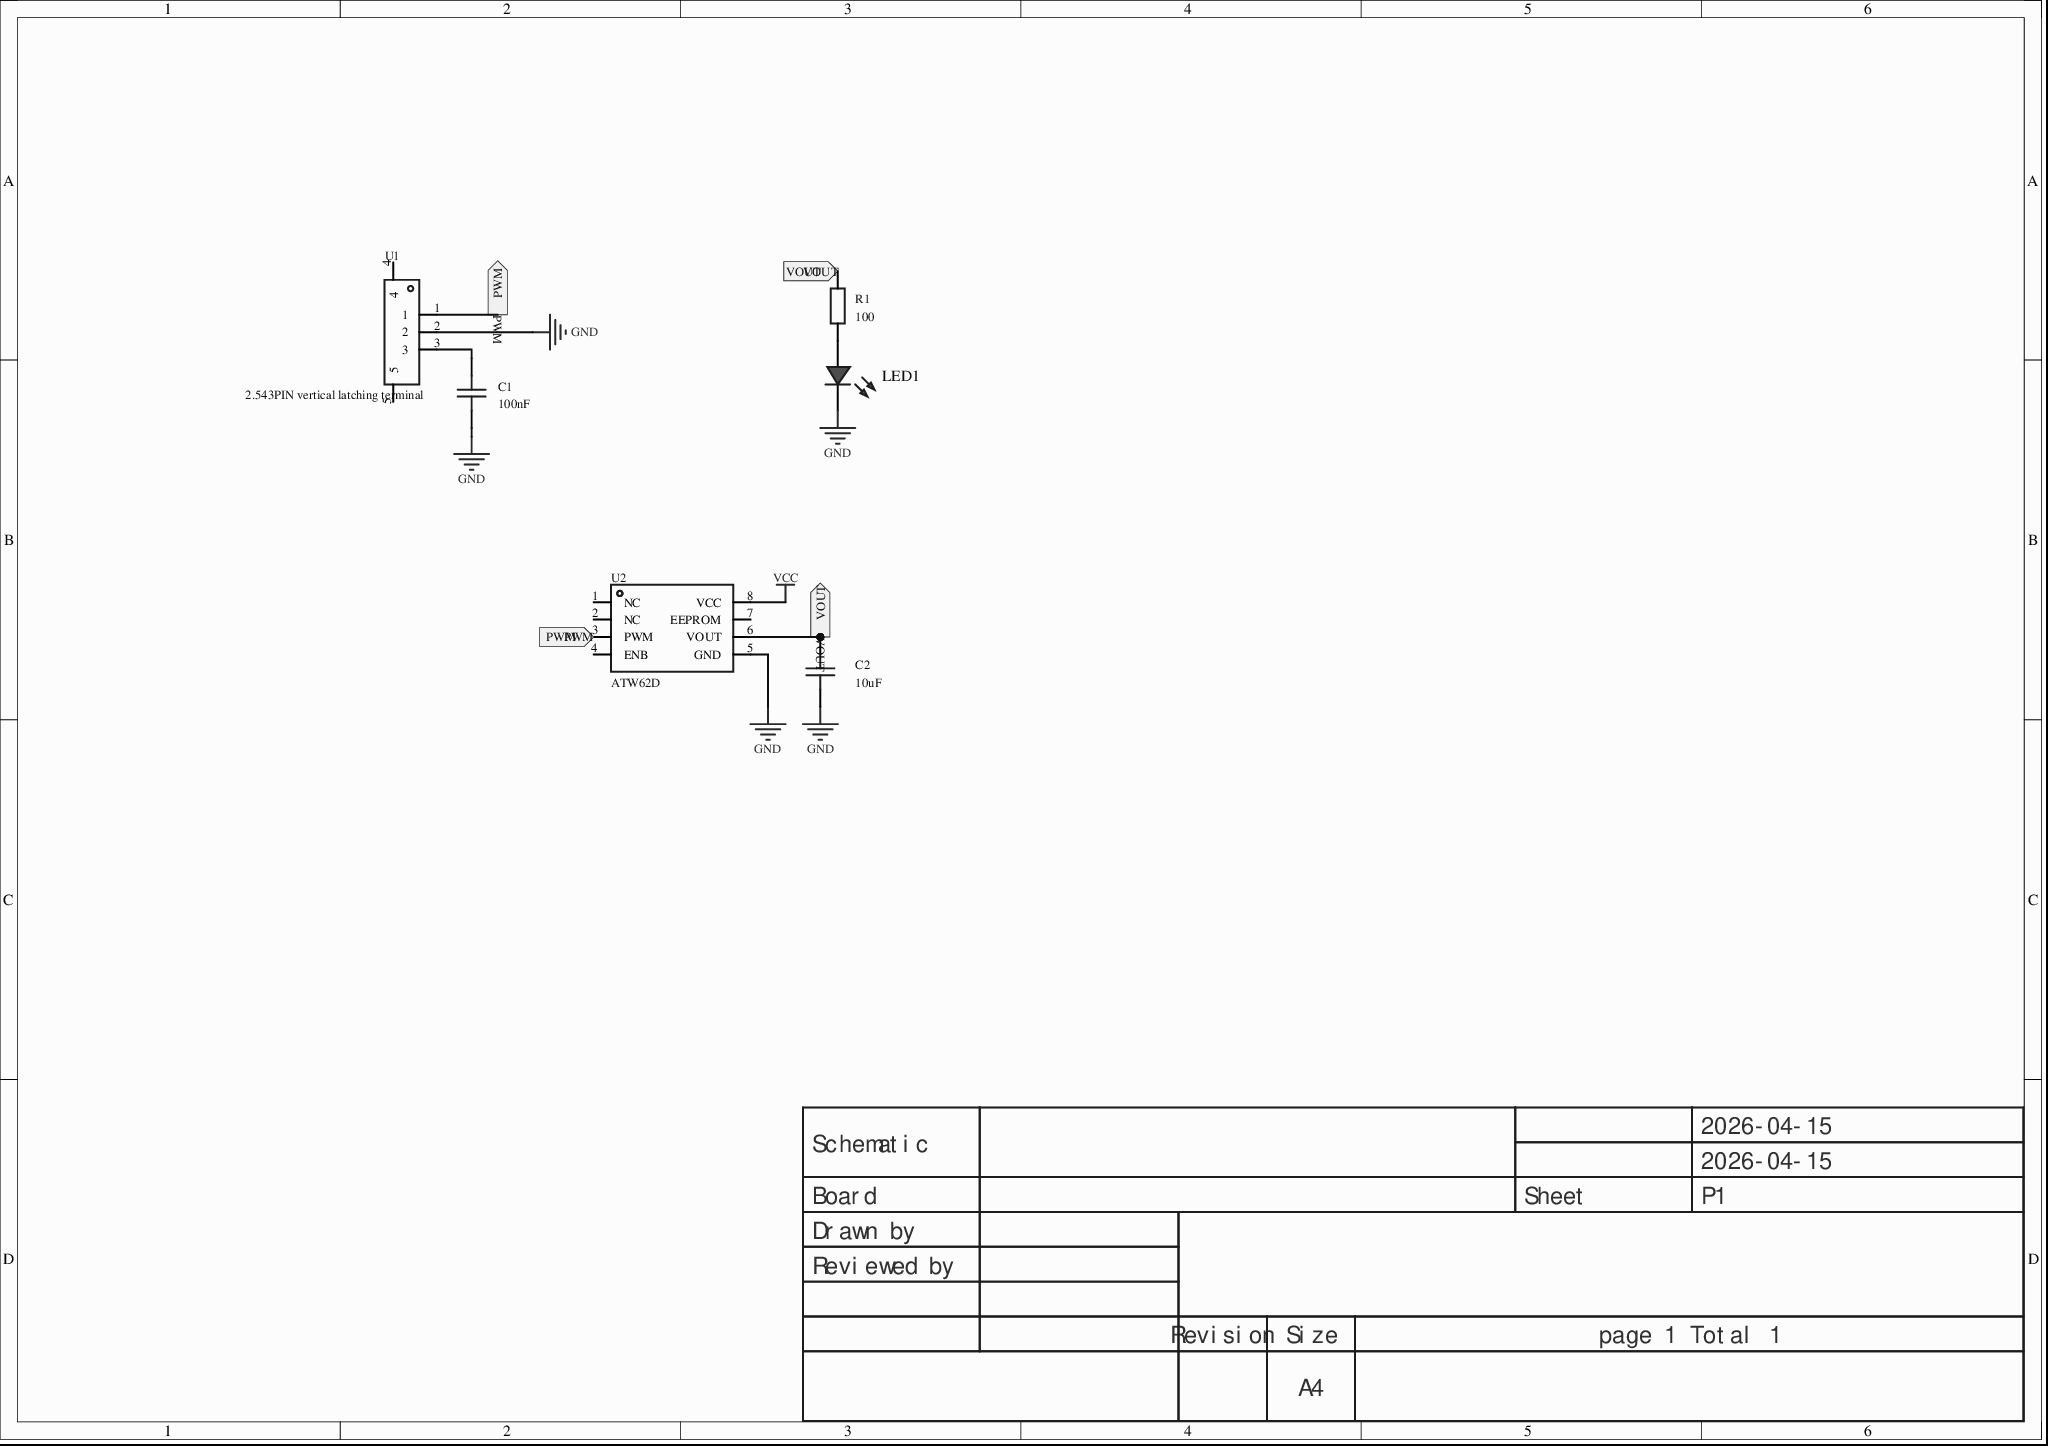
[diagram p0: MISC51135-3.schdoc]
# Altium project MISC51135-2.PrjPcb
1 sheet, 6 parts. Net scope: flat (ports and power ports of the same name join across sheets).
Board file: MISC51135.pcbdoc

## Sheet MISC51135-3.schdoc
size 297 x 209 mm; Version: V1.0; @Project Name: MISC51135; @Update Date: 2026-04-15; @Create Date: 2026-04-15; @Board Name: MISC51135; @Create Time: 19:41:14; @Page Count: 1; @Page No: 1; @Schematic Name: MISC51135; @Update Time: 19:41:14; Size: A4

### Parts
C1  100nF  [C0603]
C2  10uF  [C0603]
LED1  (no value)  [LED_0603]
R1  100  [R0603]
U1  2.543PIN vertical latching terminal  [CONN-SMD_3P-P2.54_C9900012759]
U2  ATW62D  [SOP-8_L4.9-W3.9-P1.27-LS6.0-TL]

### Ports
PWM (in), PWM (out), VOUT (in), VOUT (out)

### Nets
GND: C1.1 C2.1 LED1.1(C) U1.2 U2.5(GND)
VCC: U2.8(VCC)
PWM: U1.1 U2.3(PWM) ; port PWM
VOUT: C2.2 R1.2 U2.6(VOUT) ; port VOUT
NetC1_2: C1.2 U1.3
NetLED1_2: LED1.2(A) R1.1

Not connected (* = marked no-connect by the designer): U1 4 5; U2 1(NC)* 2(NC)* 4(ENB)* 7(EEPROM)*

### Notes on the sheet
- 2026-04-15
- Schematic
- Board
- Sheet
- P1
- Drawn by
- Reviewed by
- Revision
- Size
- A4
- page 1 Total 1

### Library data of the parts
C1 C2 = CAP_0603: Symbol: Capacitance; ConvertToPcb: yes; ModelId: ac125912035d415993ca9572d50418b10819f05c4eef4c71ace90d822a990e87; ModelName: C0603_L1.6-W0.8-H0.8; ModelTransform: 62.992,31.496,0,0,0,0,0,0,0; Device: CAP_0603; AddInBom: yes; Supplier Footprint: 0603; FootprintName: C0603
  C1: Value: 100nF
  C2: Value: 10uF
LED1 = LED_0603-R: Symbol: LED_R; Convert to PCB: yes; 3D Model: dd8257b0d61a4cd7b68939a056e080950819f05c4eef4c71ace90d822a990e87; 3D Model Transform: 58.72,29.4,22.03,0,0,0,0,0,0; ModelName: LED-0603_R; Device: LED_0603-R; Add into BOM: yes; Supplier Footprint: 0603; FootprintName: LED_0603
R1 = Res_0603: Symbol: Resistor; ConvertToPcb: yes; ModelId: fc143cca1e79419f9cd78b61e9279f080819f05c4eef4c71ace90d822a990e87; ModelTransform: 31.8897,63.7794,0,90,0,0,0,0,0; Device: Res_0603; Value: 100; AddInBom: yes; Supplier Footprint: 0603; FootprintName: R0603; ModelName: R0603
U1 = 2.543PIN立式带扣端子: AddInBom: yes; ModelId: e672aca2079f4222800d5ee53b0878840819f05c4eef4c71ace90d822a990e87; ModelTransform: 495.2746,314.96,0,180,0,0,-0.002,-5.035,0; Symbol: 2.543PIN vertical latching terminal; Device: 2.543PIN vertical latching terminal; LCSC Part Name: 2.543PIN立式带扣端子; SupplierPart: C9900012759; ManufacturerPart: 2.543PIN立式带扣端子; Supplier Footprint: XH2.54-LS-3P; JLCPCB Part Class: Extended Part; Supplier: LCSC; ConvertToPcb: yes; FootprintName: CONN-SMD_3P-P2.54_C9900012759; ModelName: CONN-SMD_3P-P2.54_C9900012759
U2 = ATW62D: Symbol: ATW62D_1; AddInBom: yes; ModelId: 4f1f5228684a45afaa7af8cce46001de0819f05c4eef4c71ace90d822a990e87; ModelName: SOP-8_L4.9-W3.9-H1.45-LS6.0-P1.27; ModelTransform: 236.22,189.751,0,0,0,0,-0.005,0.003,0; Device: ATW62D; LCSC Part Name: ATW62D; SupplierPart: C9900020806; ManufacturerPart: ATW62D; Supplier Footprint: SOP-8; JLCPCB Part Class: Extended Part; Supplier: LCSC; ConvertToPcb: yes; FootprintName: SOP-8_L4.9-W3.9-P1.27-LS6.0-TL